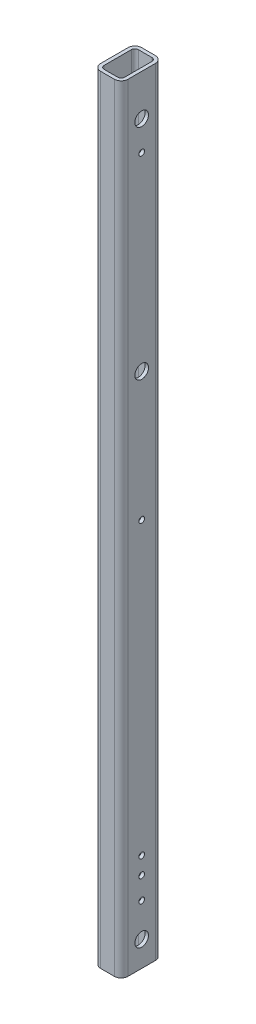
SolidWorks part; units mm, degrees
material "Q235A"
ref_plane "前视基准面" through (0, 0, 0) normal (0, 0, 1) x (1, 0, 0)
ref_plane "上视基准面" through (0, 0, 0) normal (0, 1, 0) x (1, 0, 0)
ref_plane "右视基准面" through (0, 0, 0) normal (1, 0, 0) x (0, 0, -1)
sketch "草图1" plane through (0, 0, 0) normal (0, 0, 1) x (1, 0, 0)
  line L0 (0, 0) -> (0, 568)
  dimension "D1" = 568
other "矩型管 30X20X2.5(1)"
ref_plane "基准面1" through (0, 0, 0) normal (0, 1, 0) x (-1, 0, 0)
sketch "Sketch14" plane through (0, 0, 0) normal (0, 1, 0) x (-1, 0, 0)
  line L0 (-5, -12.5) -> (5, -12.5)
  line L1 (-7.5, -10) -> (-7.5, 10)
  line L2 (5, 12.5) -> (-5, 12.5)
  line L3 (7.5, 10) -> (7.5, -10)
  line L4 (-5, -15) -> (5, -15)
  line L5 (-10, -10) -> (-10, 10)
  line L6 (5, 15) -> (-5, 15)
  line L7 (10, 10) -> (10, -10)
  arc A0 (10, 10) -> (5, 15) centre (5, 10) ccw
  arc A1 (5, -15) -> (10, -10) centre (5, -10) ccw
  arc A2 (-10, -10) -> (-5, -15) centre (-5, -10) ccw
  arc A3 (-5, 15) -> (-10, 10) centre (-5, 10) ccw
  arc A4 (-5, 12.5) -> (-7.5, 10) centre (-5, 10) ccw
  arc A5 (7.5, 10) -> (5, 12.5) centre (5, 10) ccw
  arc A6 (5, -12.5) -> (7.5, -10) centre (5, -10) ccw
  arc A7 (-7.5, -10) -> (-5, -12.5) centre (-5, -10) ccw
  point P0 (0, 15)
  point P1 (10, 0)
  point P2 (0, -15)
  point P3 (-10, 0)
  point P4 (-10, 15)
  point P5 (10, 15)
  point P6 (10, -15)
  point P7 (-10, -15)
  point P8 (0, 0)
  point P33 (0, 0)
sketch "草图6" plane through (-10, 0, 0) normal (-1, 0, 0) x (0, 0, 1)
  line L1 (-10, 0) -> (10, 0) construction
  circle A0 centre (0, 18.5) radius 10.5
  dimension "D1" = 21
  dimension "D2" = 8
extrude "切除-拉伸1" cut sketch "草图6" against normal up to next
hole_wizard "M8 间隙孔1" positions "草图7" profile "草图8" hole size "M8" standard "ISO" end condition through all
sketch "草图7" plane through (-10, 0, 0) normal (-1, 0, 0) x (0, 0, 1)
  point P0 (0, 538)
  point P3 (0, 378)
  point P6 (0, 18.5)
sketch "草图8" plane through (-10, 538, 0) normal (0, 1, 0) x (0, 0, 1)
  line L0 (0, 0) -> (0, 20)
  line L1 (0, 20) -> (5, 20)
  line L2 (5, 20) -> (5, 0)
  line L5 (5, 0) -> (0, 0)
  line L11 (0, -6.35) -> (0, 107.95) construction
  dimension "通孔孔直径" = 10
  dimension "通孔孔深度" = 20
hole_wizard "M5 螺纹孔1" positions "草图9" profile "草图10" tap size "M5" standard "ISO" end condition through all
sketch "草图9" plane through (10, 0, 0) normal (1, 0, 0) x (0, 0, -1)
  line L0 (-10, 284) -> (10, 284) construction
  line L1 (-10, 568) -> (-10, 0) construction
  line L2 (10, 568) -> (10, 0) construction
  line L4 (-10, 568) -> (10, 568) construction
  arc A1 (10, 21.7016) -> (-10, 21.7016) centre (0, 18.5) ccw construction
  point P0 (0, 516.5)
  point P2 (0, 284)
  point P4 (0, 71.5)
  point P21 (0, 59)
  point P31 (0, 43)
  dimension "D1" = 51.5
  dimension "D2" = 71.5
  dimension "D3" = 30
  dimension "D4" = 16
sketch "草图10" plane through (10, 516.5, 0) normal (0, 1, 0) x (0, 0, -1)
  line L0 (0, 0) -> (0, 20)
  line L1 (0, 20) -> (2.1, 20)
  line L2 (2.1, 20) -> (2.1, 0)
  line L5 (2.1, 0) -> (0, 0)
  line L11 (0, -6.35) -> (0, 107.95) construction
  dimension "通孔螺纹孔钻头直径" = 4.2
  dimension "通孔螺纹孔钻头深度" = 20
cosmetic thread "孔螺蚊线1" parameters "D2"=5
cosmetic thread "孔螺蚊线2" parameters "D2"=5
cosmetic thread "孔螺蚊线3" parameters "D2"=5
cosmetic thread "孔螺蚊线4" parameters "D2"=5
cosmetic thread "孔螺蚊线5" parameters "D2"=5
equation "\"D1@Sketch14\"= \"Thickness@Sketch14\" * 2"
